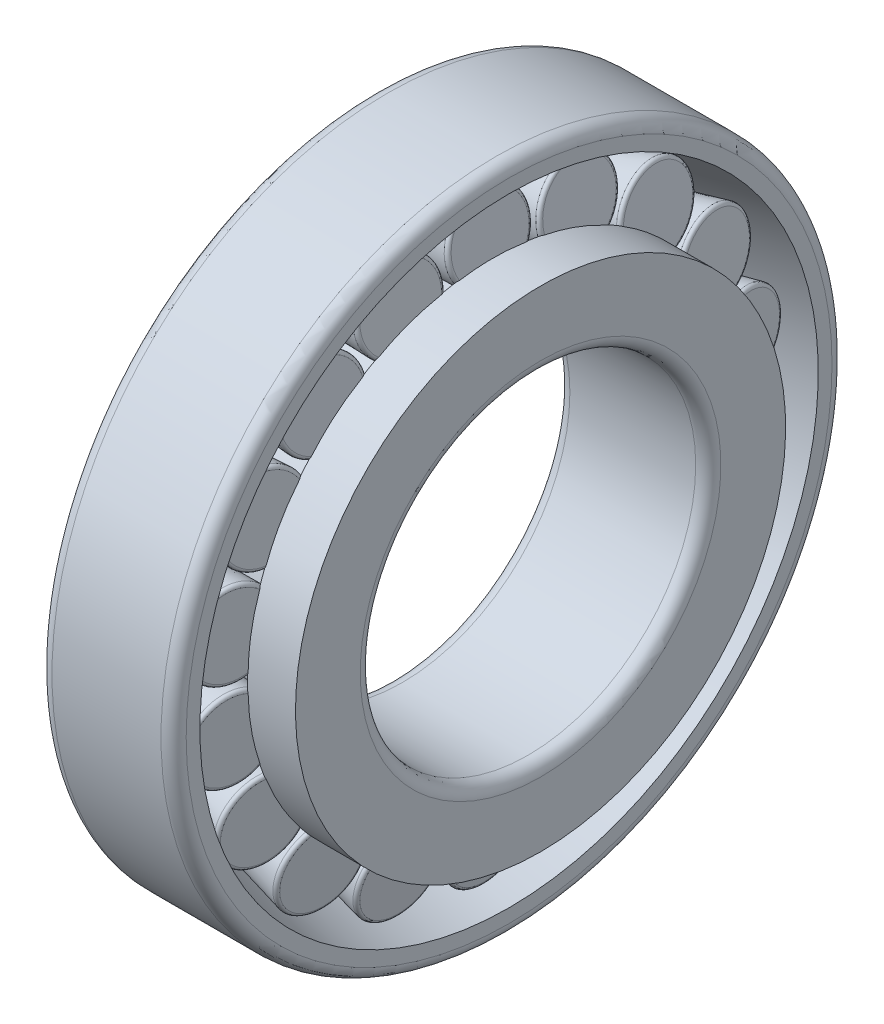
SolidWorks part; units mm, degrees
ref_plane "Front" through (0, 0, 0) normal (0, 0, 1) x (1, 0, 0)
ref_plane "Top" through (0, 0, 0) normal (0, 1, 0) x (1, 0, 0)
ref_plane "Right" through (0, 0, 0) normal (1, 0, 0) x (0, 0, -1)
sketch "Sketch1" plane through (0, 0, 0) normal (0, 0, 1) x (1, 0, 0)
  line L0 (11.75, 0) -> (13.9916, 0) construction
  line L1 (8, 36.8649) -> (8, 38.5)
  line L2 (6.5, 40) -> (-6.5, 40)
  line L3 (-8, 38.5) -> (-8, 32.865)
  line L4 (-8, 32.865) -> (8, 36.8649)
  line L5 (-6.25, 21.5) -> (-6.25, 26.982)
  line L6 (-4.75, 20) -> (10.25, 20)
  line L7 (11.75, 21.5) -> (11.75, 29.2214)
  line L8 (-3.9796, 25.482) -> (-5.2625, 33.5494)
  line L9 (6.5, 26.2214) -> (4.9294, 36.0973)
  line L10 (-4.621, 29.5157) -> (5.7147, 31.1594) construction
  line L11 (-3.9796, 25.482) -> (6.5, 26.2214)
  line L12 (6.0229, 30) -> (11.75, 30)
  line L13 (11.75, 29.2214) -> (6.0229, 29.2214)
  line L14 (-6.25, 26.982) -> (-4.2181, 26.982)
  arc A0 (-6.5, 40) -> (-8, 38.5) centre (-6.5, 38.5) ccw
  arc A1 (8, 38.5) -> (6.5, 40) centre (6.5, 38.5) ccw
  arc A2 (-4.75, 20) -> (-6.25, 21.5) centre (-4.75, 21.5) cw
  arc A3 (10.25, 20) -> (11.75, 21.5) centre (10.25, 21.5) ccw
  point P19 (-8, 40)
  point P22 (8, 40)
  point P24 (0, 40)
  point P29 (-6.25, 20)
  point P32 (11.75, 20)
revolve "Revolve1" add sketch "Sketch1" angle 360 about L0
sketch "Sketch2" plane through (0, 0, 0) normal (0, 0, 1) x (1, 0, 0)
  line L0 (-4.6408, 29.5125) -> (8.1583, 31.5479) construction
  line L4 (-4.621, 29.5157) -> (5.7147, 31.1594) construction
  line L5 (-4.6408, 29.5125) -> (5.7345, 31.1625)
  line L7 (-5.2823, 33.5462) -> (-3.9964, 25.4607)
  line L8 (6.5232, 26.203) -> (4.9492, 36.1004)
  line L9 (-3.9964, 25.4607) -> (6.5232, 26.203)
  line L10 (-4.6408, 29.5125) -> (-4.054, 25.8227)
  line L11 (6.4546, 26.6341) -> (5.7345, 31.1625)
  line L12 (-3.6308, 25.4865) -> (6.0877, 26.1723)
  arc A0 (-3.6308, 25.4865) -> (-4.054, 25.8227) centre (-3.659, 25.8856) cw
  arc A1 (6.0877, 26.1723) -> (6.4546, 26.6341) centre (6.0596, 26.5713) ccw
revolve "Revolve2" add sketch "Sketch2" angle 360 about L0
sketch "Sketch3" plane through (0, 0, 0) normal (0, 0, 1) x (1, 0, 0)
  line L0 (-8, 32.865) -> (8, 36.8649) construction
  line L1 (-8, 38.5) -> (-8, 32.865) construction
  line L2 (6.5, 40) -> (-6.5, 40) construction
  line L3 (8, 36.8649) -> (8, 38.5) construction
  line L4 (-8, 32.865) -> (8, 36.8649)
  line L5 (-8, 38.5) -> (-8, 32.865)
  line L6 (6.5, 40) -> (-6.5, 40)
  line L7 (8, 36.8649) -> (8, 38.5)
  arc A0 (-6.5, 40) -> (-8, 38.5) centre (-6.5, 38.5) ccw construction
  arc A1 (8, 38.5) -> (6.5, 40) centre (6.5, 38.5) ccw construction
  arc A2 (-6.5, 40) -> (-8, 38.5) centre (-6.5, 38.5) ccw
  arc A3 (8, 38.5) -> (6.5, 40) centre (6.5, 38.5) ccw
revolve "Revolve3" add sketch "Sketch3" angle 360 about axis through (11.75, 0, 0) along (1, 0, 0)
pattern_circular "Circular-Pattern1" count 18 over 360 about axis through (0, 0, 0) along (1, 0, 0) of "Revolve2"
equation "\"gzzj@Sketch1\" =  ( \"DD@Sketch1\" - \"XD@Sketch1\" )  / 4"
equation "\"D1@Sketch1\" = \"DB@Sketch1\" - \"DT@Sketch1\" / 20"
equation "\"D2@Sketch1\" = \"DT@Sketch1\" - \"DC@Sketch1\" + \"XR12@Sketch1\""
equation "\"D4@Sketch1\" = \"D3@Sketch1\" / 2"
equation "\"D2@Sketch2\" = \"gzzj@Sketch1\" / 25"
equation "\"ZJ@Sketch1\" =  ( \"DD@Sketch1\" + \"XD@Sketch1\" )  / 2"
equation "\"D1@Circular-Pattern1\" = int( 3.14159265 / atn(( \"gzzj@Sketch1\" / 2) / sqr( \"ZJ@Sketch1\" * \"ZJ@Sketch1\" /4 - ( \"gzzj@Sketch1\"/ 2) *  ( \"gzzj@Sketch1\"/ 2))))"
